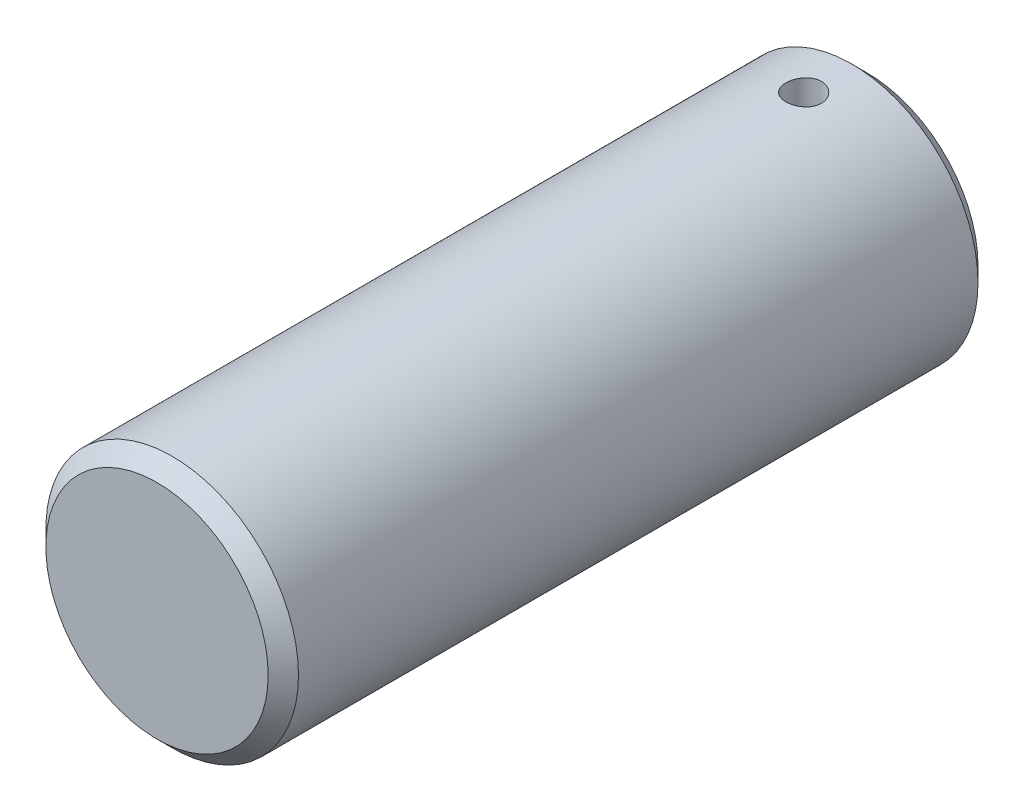
SolidWorks part; units mm, degrees
material "AISI 1020"
ref_plane "Front Plane" through (0, 0, 0) normal (0, 0, 1) x (1, 0, 0)
ref_plane "Top Plane" through (0, 0, 0) normal (0, 1, 0) x (1, 0, 0)
ref_plane "Right Plane" through (0, 0, 0) normal (1, 0, 0) x (0, 0, -1)
sketch "Sketch1" plane through (0, 0, 0) normal (0, 0, 1) x (1, 0, 0)
  circle A0 centre (0, 0) radius 12.7
  dimension "D1" = 25.4
extrude "Boss-Extrude1" add sketch "Sketch1" along normal blind 71.37
chamfer "Chamfer1" distance 1.524 angle 45 2 edges at (12.7, 0, 0) (12.7, 0, 71.37)
sketch "Sketch2" plane through (0, 0, 0) normal (0, 1, 0) x (1, 0, 0)
  line L0 (0, 0) -> (0, -21.9498) construction
  line L1 (-15.0799, -6.35) -> (14.2155, -6.35) construction
  line L2 (11.176, 0) -> (-11.176, 0) construction
  circle A0 centre (0, -6.35) radius 1.785
  dimension "D2" = 3.57
  dimension "D1" = 6.35
extrude "Cut-Extrude1" cut sketch "Sketch2" against normal through all and the other way through all
